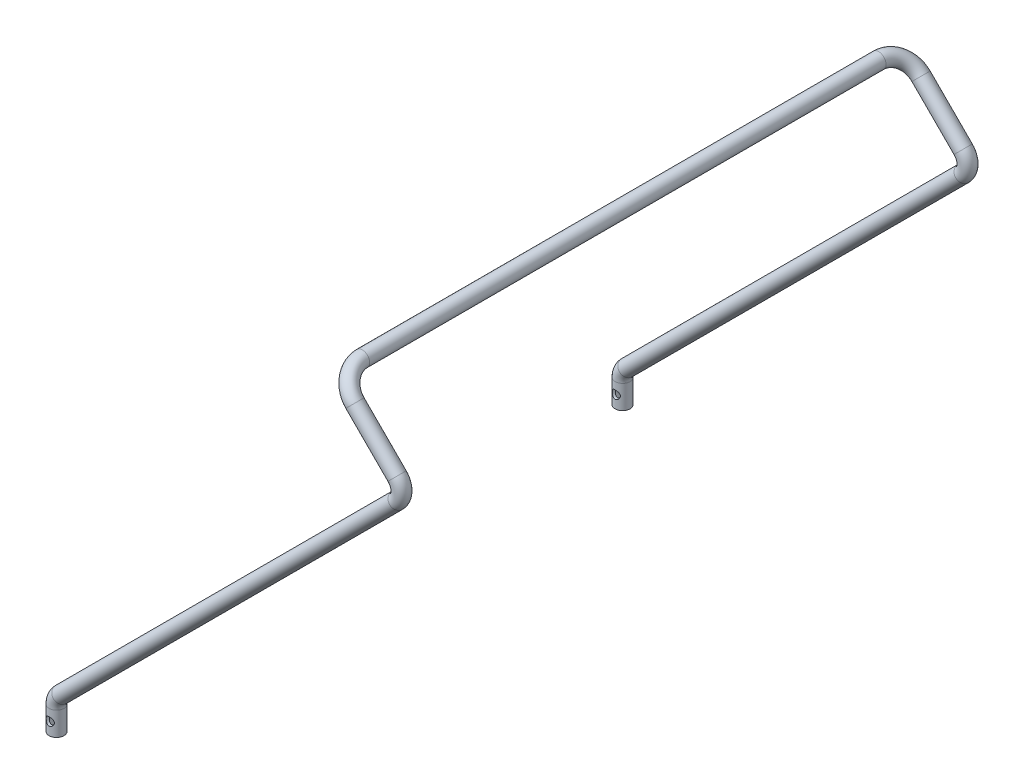
SolidWorks part; units mm, degrees
ref_plane "Front Plane" through (0, 0, 0) normal (0, 0, 1) x (1, 0, 0)
ref_plane "Top Plane" through (0, 0, 0) normal (0, 1, 0) x (1, 0, 0)
ref_plane "Right Plane" through (0, 0, 0) normal (1, 0, 0) x (0, 0, -1)
ref_plane "Plane1" through (0, 0, 570) normal (0, 0, 1) x (1, 0, 0)
sketch "Sketch2" plane through (0, 0, 570) normal (0, 0, 1) x (1, 0, 0)
  line L0 (0, 0) -> (0, 47.5736)
  line L1 (8.7868, 68.7868) -> (685.8936, 745.8936)
  line L2 (685.8936, 788.32) -> (565.6854, 908.5281)
  arc A0 (0, 47.5736) -> (8.7868, 68.7868) centre (30, 47.5736) cw
  arc A1 (685.8936, 788.32) -> (685.8936, 745.8936) centre (664.6804, 767.1068) cw
  point P6 (0, 60)
  point P10 (707.1068, 767.1068)
  dimension "D4" = 30
  dimension "D6" = 30
  dimension "D1" = 60
  dimension "D2" = 135
  dimension "D3" = 1000
  dimension "D5" = 200
ref_plane "Plane2" through (0, 0, -570) normal (0, 0, 1) x (1, 0, 0)
sketch "Sketch3" plane through (0, 0, -570) normal (0, 0, 1) x (1, 0, 0)
  line L0 (0, 0) -> (0, 47.5736) construction
  line L1 (8.7868, 68.7868) -> (685.8936, 745.8936) construction
  line L2 (0, 0) -> (0, 47.5736)
  line L3 (8.7868, 68.7868) -> (685.8936, 745.8936)
  line L4 (685.8936, 788.32) -> (565.6854, 908.5281) construction
  line L5 (685.8936, 788.32) -> (565.6854, 908.5281)
  arc A0 (8.7868, 68.7868) -> (0, 47.5736) centre (30, 47.5736) ccw construction
  arc A1 (8.7868, 68.7868) -> (0, 47.5736) centre (30, 47.5736) ccw
  arc A2 (685.8936, 745.8936) -> (685.8936, 788.32) centre (664.6804, 767.1068) ccw construction
  arc A3 (685.8936, 745.8936) -> (685.8936, 788.32) centre (664.6804, 767.1068) ccw
sketch3d "3DSketch3"
  line L0 (565.6854, 908.5281, -570) -> (565.6854, 908.5281, 570)
sketch3d "3DSketch4"
  line L0 (0, 0, 570) -> (0, 47.5736, 570) construction
  line L1 (8.7868, 68.7868, 570) -> (685.8936, 745.8936, 570) construction
  line L2 (685.8936, 788.32, 570) -> (565.6854, 908.5281, 570) construction
  line L3 (565.6854, 908.5281, -570) -> (565.6854, 908.5281, 570) construction
  line L4 (685.8936, 788.32, -570) -> (565.6854, 908.5281, -570) construction
  line L5 (8.7868, 68.7868, -570) -> (685.8936, 745.8936, -570) construction
  line L6 (0, 0, -570) -> (0, 47.5736, -570) construction
  line L7 (0, 0, 570) -> (0, 47.5736, 570)
  line L8 (8.7868, 68.7868, 570) -> (685.8936, 745.8936, 570)
  line L9 (685.8936, 788.32, 570) -> (601.0408, 873.1728, 570)
  line L10 (565.6854, 908.5281, -520) -> (565.6854, 908.5281, 520)
  line L11 (685.8936, 788.32, -570) -> (601.0408, 873.1728, -570)
  line L12 (8.7868, 68.7868, -570) -> (685.8936, 745.8936, -570)
  line L13 (0, 0, -570) -> (0, 47.5736, -570)
  arc A0 (0, 47.5736, 570) -> (8.7868, 68.7868, 570) centre (30, 47.5736, 570) ccw construction
  arc A1 (685.8936, 788.32, 570) -> (685.8936, 745.8936, 570) centre (664.6804, 767.1068, 570) ccw construction
  arc A2 (685.8936, 745.8936, -570) -> (685.8936, 788.32, -570) centre (664.6804, 767.1068, -570) ccw construction
  arc A3 (8.7868, 68.7868, -570) -> (0, 47.5736, -570) centre (30, 47.5736, -570) ccw construction
  arc A4 (0, 47.5736, 570) -> (8.7868, 68.7868, 570) centre (30, 47.5736, 570) ccw
  arc A5 (685.8936, 788.32, 570) -> (685.8936, 745.8936, 570) centre (664.6804, 767.1068, 570) ccw
  arc A6 (685.8936, 745.8936, -570) -> (685.8936, 788.32, -570) centre (664.6804, 767.1068, -570) ccw
  arc A7 (8.7868, 68.7868, -570) -> (0, 47.5736, -570) centre (30, 47.5736, -570) ccw
  arc A8 (601.0408, 873.1728, 570) -> (565.6854, 908.5281, 520) centre (601.0408, 873.1728, 520) ccw
  arc A9 (565.6854, 908.5281, -520) -> (601.0408, 873.1728, -570) centre (601.0408, 873.1728, -520) ccw
  point P3 (30, 47.5736, 540)
  point P5 (30, 47.5736, 540)
  point P6 (664.6804, 767.1068, 540)
  point P10 (664.6804, 767.1068, -540)
  point P11 (664.6804, 767.1068, 540)
  point P12 (30, 47.5736, -540)
  point P20 (565.6854, 908.5281, 570)
  point P21 (664.6804, 767.1068, -540)
  point P25 (565.6854, 837.8175, 520)
  point P27 (30, 47.5736, -540)
  point P31 (565.6854, 908.5281, -570)
  point P33 (565.6854, 837.8175, -520)
  dimension "D1" = 50
sweep "Sweep1" add path "3DSketch4" circular profile diameter 30 parameters "D3"=30
shell "Shell1" thickness 5
sketch "Sketch4" plane through (0, 0, 0) normal (0, 0, 1) x (1, 0, 0)
  circle A0 centre (0, 25) radius 8.1928
extrude "Cut-Extrude1" cut sketch "Sketch4" against normal through all both and the other way through all
